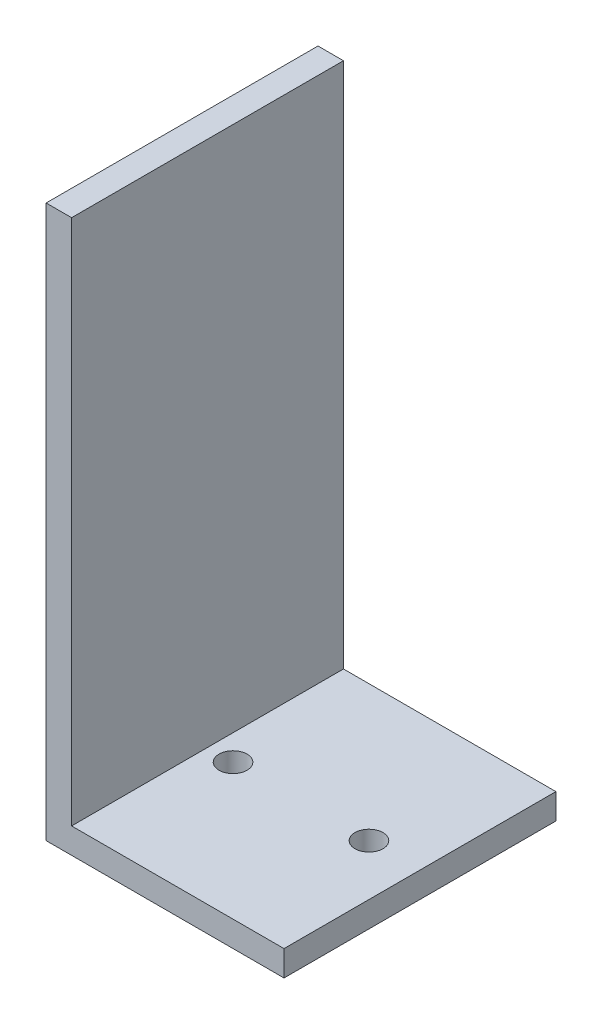
from build123d import *

# Parameters (mm, degrees)
EXTRUDE_1_DEPTH     = 16
SKETCH_2_R          = 1.65
CUT_EXTRUDE_1_DEPTH = 7.5


with BuildPart() as part:
    # 草图1 → 凸台-拉伸1 (new, symmetric)
    with BuildSketch(Plane.XY):
        Polygon((0, 0), (28, 0), (28, 3), (3, 3), (3, 65), (0, 65), align=None)
    extrude(amount=EXTRUDE_1_DEPTH, both=True)

    # 草图2 → 切除-拉伸1 (cut, symmetric)
    with BuildSketch(Plane(origin=(0, 0, 0), x_dir=(1, 0, 0), z_dir=(0, 1, 0))):
        with Locations(Location((6, 0, 0), (0, 0, 270))):
            Circle(SKETCH_2_R)
        with Locations(Location((22, 0, 0), (0, 0, 270))):
            Circle(SKETCH_2_R)
    extrude(amount=CUT_EXTRUDE_1_DEPTH, both=True, mode=Mode.SUBTRACT)


solid = part.part
